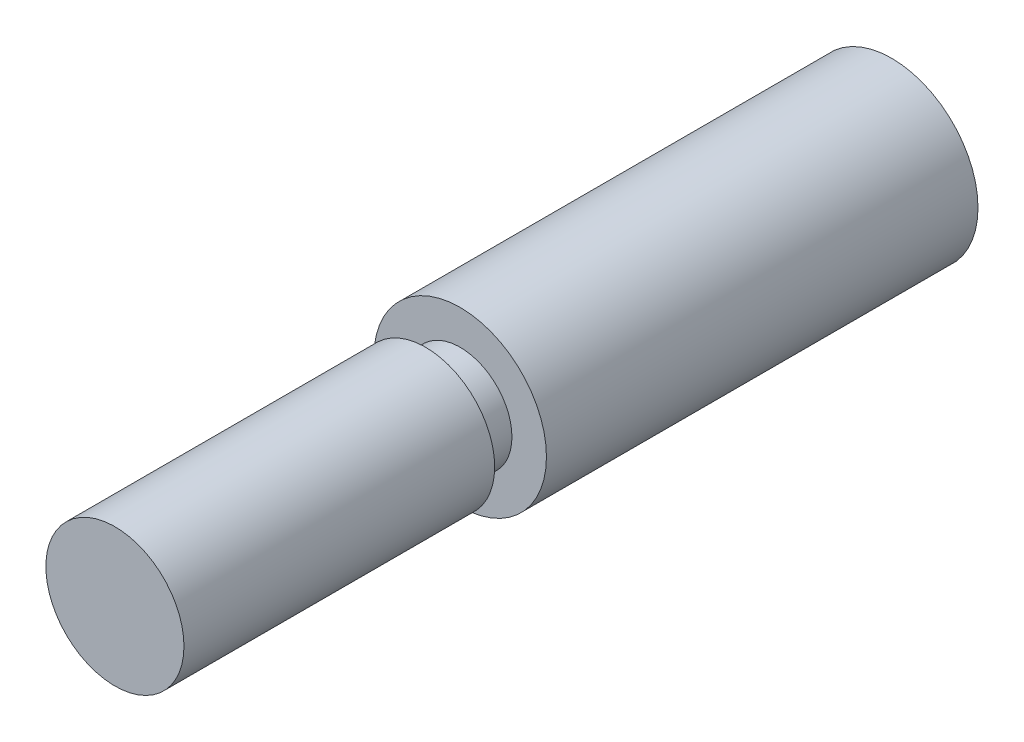
from build123d import *

# Parameters (mm, degrees)
SKETCH1_R           = 5
BOSS_EXTRUDE1_DEPTH = 25
SKETCH2_R           = 4
BOSS_EXTRUDE2_DEPTH = 20
SKETCH3_OUTSIDE_W   = 21.434
SKETCH3_OUTSIDE_H   = 21.434
SKETCH3_OUTSIDE_R   = 3
CUT_EXTRUDE1_DEPTH  = 2


with BuildPart() as part:
    # Sketch1 → Boss-Extrude1 (new body)
    with BuildSketch(Plane.XY):
        Circle(SKETCH1_R)
    extrude(amount=BOSS_EXTRUDE1_DEPTH)

    # Sketch2 → Boss-Extrude2 (add)
    with BuildSketch(Plane.XY.offset(25)):
        Circle(SKETCH2_R)
    extrude(amount=BOSS_EXTRUDE2_DEPTH)

    # Sketch3 outside → Cut-Extrude1 (cut)
    with BuildSketch(Plane.XY.offset(25)):
        Rectangle(SKETCH3_OUTSIDE_W, SKETCH3_OUTSIDE_H)
        Circle(SKETCH3_OUTSIDE_R, mode=Mode.SUBTRACT)
    extrude(amount=CUT_EXTRUDE1_DEPTH, mode=Mode.SUBTRACT)


solid = part.part
